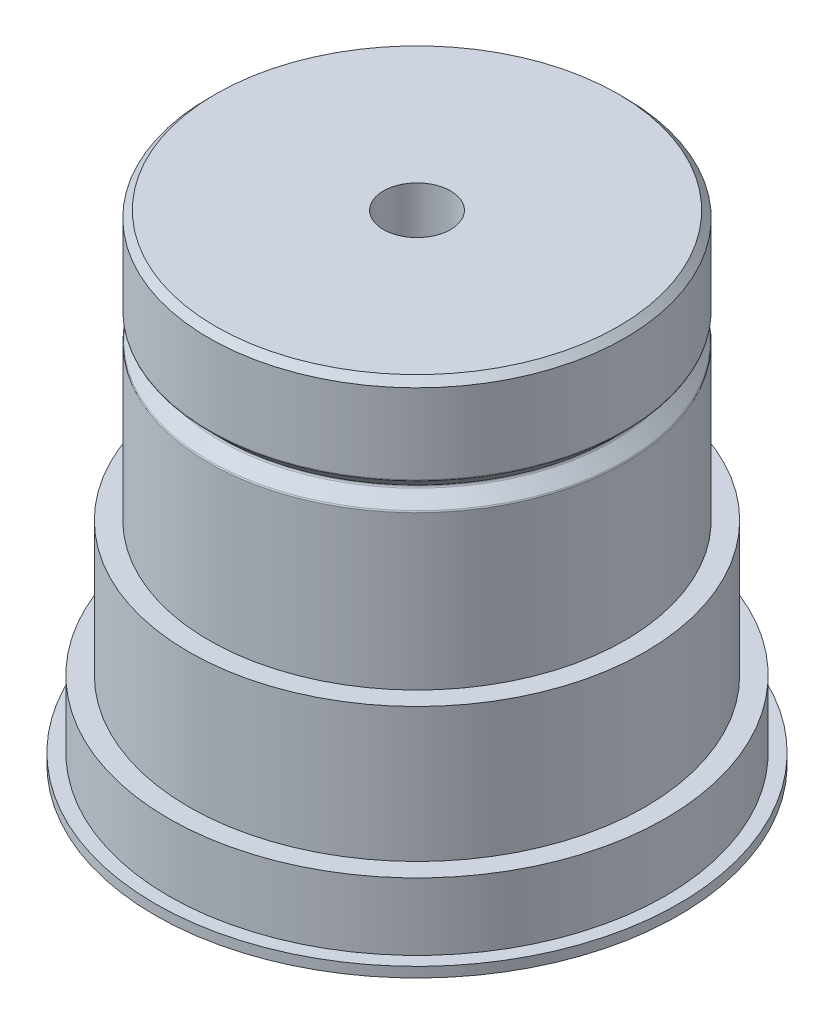
from build123d import *

# Parameters (mm, degrees)
CHAMFER_1_SIZE = 1


with BuildPart() as part:
    # 草图1 → 旋转1 (revolve)
    with BuildSketch(Plane.XY, mode=Mode.PRIVATE) as revolve_1_sk:
        with BuildLine():
            Line((-12.5, 0), (-12.5, 25))
            Line((-12.5, 25), (-5, 25))
            Line((-5, 25), (-5, 71.5))
            Line((-5, 71.5), (-31, 71.5))
            Line((-31, 71.5), (-31, 58.624264069))
            ThreePointArc((-31, 58.624264069), (-30.97716386, 58.509459039), (-30.912132034, 58.412132034))
            Line((-30.912132034, 58.412132034), (-29.212132034, 56.712132034))
            ThreePointArc((-29.212132034, 56.712132034), (-29.124264069, 56.5), (-29.212132034, 56.287867966))
            Line((-29.212132034, 56.287867966), (-30.912132034, 54.587867966))
            ThreePointArc((-30.912132034, 54.587867966), (-30.97716386, 54.490540961), (-31, 54.375735931))
            Line((-31, 54.375735931), (-31, 31.5))
            Line((-31, 31.5), (-34, 31.5))
            Line((-34, 31.5), (-34, 11.5))
            Line((-34, 11.5), (-37, 11.5))
            Line((-37, 11.5), (-37, 1.5))
            Line((-37, 1.5), (-39, 1.5))
            Line((-39, 1.5), (-39, 0))
            Line((-39, 0), (-12.5, 0))
        make_face()
    revolve(revolve_1_sk.sketch.rotate(Axis((0, 0, 0), (0, 1, 0)), 270), axis=Axis((0, 0, 0), (0, 1, 0)))

    # 倒角1
    chamfer_1_edges = [part.edges().sort_by_distance(p)[0] for p in [
        (0, 71.5, 31),
    ]]
    chamfer(chamfer_1_edges, length=CHAMFER_1_SIZE)


solid = part.part
